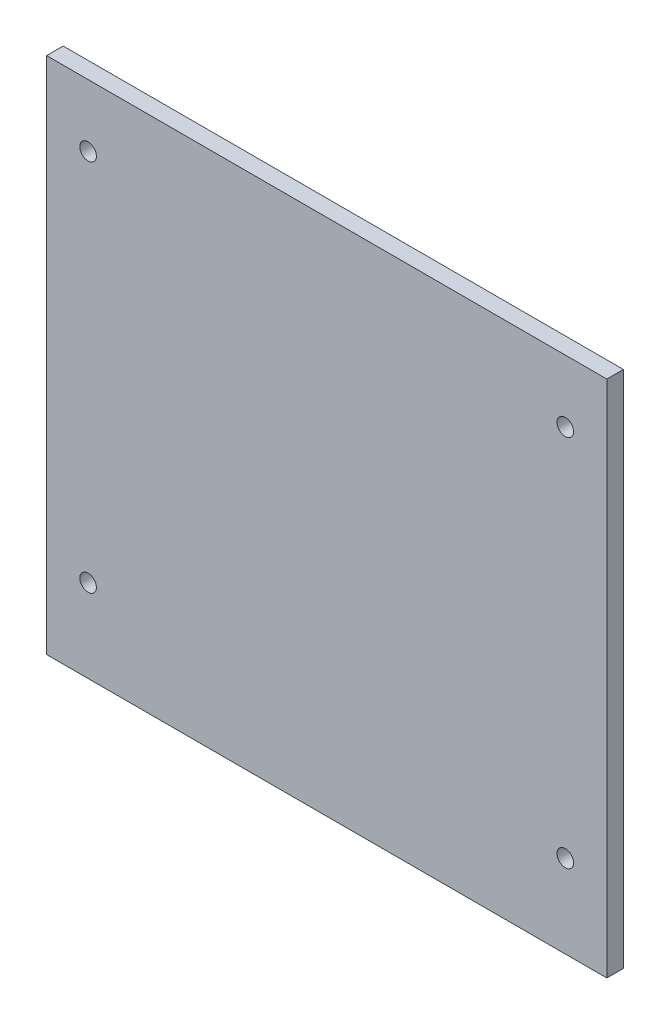
from build123d import *

# Parameters (mm, degrees)
SKETCH_1_W          = 270
SKETCH_1_H          = 250
EXTRUDE_1_DEPTH     = 8
SKETCH_2_R          = 4
CUT_EXTRUDE_1_DEPTH = 10


with BuildPart() as part:
    # 草图1 → 凸台-拉伸1 (new body)
    with BuildSketch(Plane.XY):
        with Locations((135, -125)):
            Rectangle(SKETCH_1_W, SKETCH_1_H)
    extrude(amount=EXTRUDE_1_DEPTH)

    # 草图2 → 切除-拉伸1 (cut)
    with BuildSketch(Plane.XY.offset(8)):
        with Locations((250, -30)):
            Circle(SKETCH_2_R)
        with Locations((250, -210)):
            Circle(SKETCH_2_R)
        with Locations((20, -210)):
            Circle(SKETCH_2_R)
        with Locations((20, -30)):
            Circle(SKETCH_2_R)
    extrude(amount=-CUT_EXTRUDE_1_DEPTH, mode=Mode.SUBTRACT)


solid = part.part
